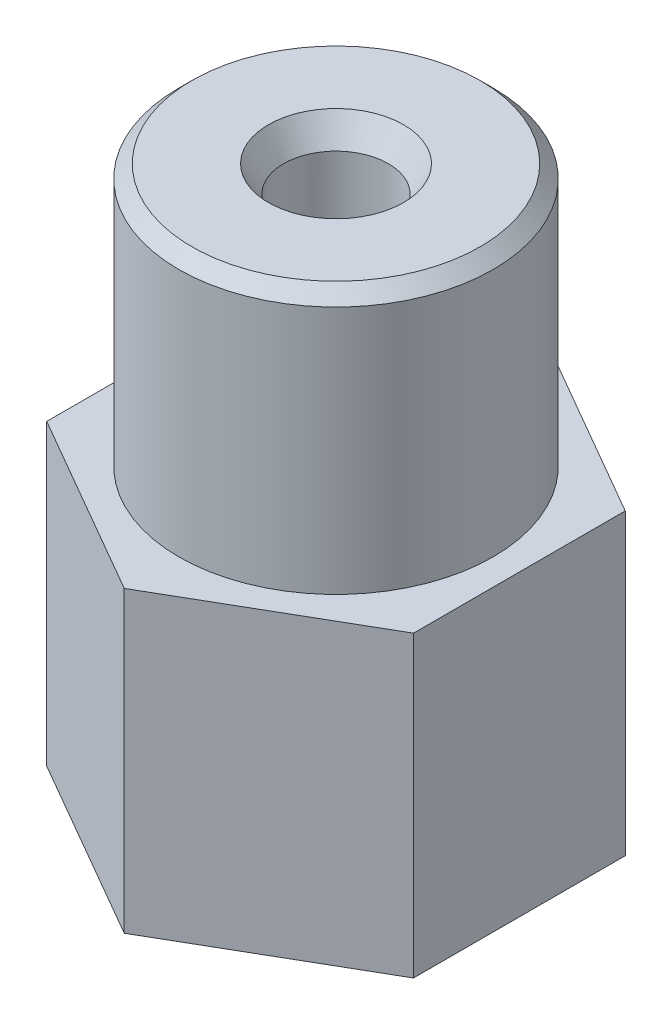
from build123d import *

# Parameters (mm, degrees)
BOSS_EXTRUDE1_DEPTH = 5.7


with BuildPart() as part:
    # Sketch1 → Revolve1 (revolve)
    with BuildSketch(Plane.XY, mode=Mode.PRIVATE) as revolve1_sk:
        Polygon((0.2, 0), (0.375, 0), (1.414230485, 1.8), (2.5, 1.8), (2.5, 6.5), (3, 7.366025404), (3, 12.25), (2.75, 12.5), (1.288675135, 12.5), (1, 12), (1, 3.985640646), (0.5, 3.119615242), (0.5, 1.119615242), (0.2, 0.6), align=None)
    revolve(revolve1_sk.sketch.rotate(Axis((0, 0, 0), (0, 1, 0)), 90), axis=Axis((0, 0, 0), (0, 1, 0)))

    # Sketch2 → Boss-Extrude1 (add)
    with BuildSketch(Plane.XZ.offset(-1.8)):
        Polygon((0, 4.041451884), (-3.5, 2.020725942), (-3.5, -2.020725942), (0, -4.041451884), (3.5, -2.020725942), (3.5, 2.020725942), align=None)
    extrude(amount=-BOSS_EXTRUDE1_DEPTH)


solid = part.part
